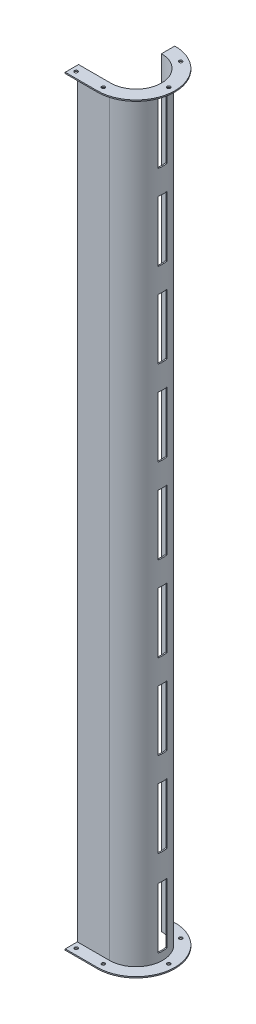
SolidWorks part; units mm, degrees
ref_plane "前视" through (0, 0, 0) normal (0, 0, 1) x (1, 0, 0)
ref_plane "上视" through (0, 0, 0) normal (0, 1, 0) x (1, 0, 0)
ref_plane "右视" through (0, 0, 0) normal (1, 0, 0) x (0, 0, -1)
sketch "草图1" plane through (0, 0, 0) normal (0, 1, 0) x (1, 0, 0)
  line L0 (0, 0) -> (59.4065, 0) construction
  line L1 (0, 0) -> (0, 69.9008) construction
  line L2 (0, 0) -> (53, 0)
  line L3 (53, 0) -> (53, 88.0268) construction
  line L4 (0, -2) -> (53, -2)
  line L5 (53, 86) -> (53, 84)
  line L6 (0, 0) -> (0, -2)
  arc A0 (53, 0) -> (53, 84) centre (53, 42) ccw
  arc A1 (53, -2) -> (53, 86) centre (53, 42) ccw
  point P6 (42.0774, 56.8644)
  point P8 (0, 44)
  point P9 (40.1648, 56.2796)
  point P10 (0, 44)
  dimension "D3" = 2
  dimension "D2" = 42
  dimension "D1" = 53
extrude "凸台-拉伸1" add sketch "草图1" along normal blind 1256
sketch "草图3" plane through (0, 1256, 0) normal (0, 1, 0) x (1, 0, 0)
  line L0 (0, 0) -> (91.5194, 0) construction
  line L1 (0, 0) -> (53, 0)
  line L2 (53, 84) -> (53, 106)
  line L4 (0, -22) -> (53, -22)
  line L5 (0, 0) -> (0, -22)
  line L6 (54.8577, 105.973) -> (43.3453, 107.7442) construction
  line L7 (53, 84) -> (40, 86) construction
  arc A0 (53, 0) -> (53, 84) centre (53, 42) ccw
  arc A1 (53, -22) -> (53, 106) centre (53, 42) ccw
  arc A2 (53, -22) -> (54.8577, 105.973) centre (53, 42) ccw construction
  dimension "D1" = 22
extrude "凸台-拉伸2" add sketch "草图3" against normal blind 2
sketch "草图4" plane through (0, 0, 0) normal (0, -1, 0) x (1, 0, 0)
  line L0 (53, 0) -> (0, 0) construction
  line L1 (53, -106) -> (53, -86) construction
  line L2 (53, -86) -> (53, -84) construction
  line L3 (0, 22) -> (53, 22) construction
  line L4 (0, 2) -> (0, 22) construction
  line L5 (0, 0) -> (0, 2) construction
  line L6 (53, 0) -> (0, 0)
  line L7 (53, -106) -> (53, -86)
  line L8 (53, -86) -> (53, -84)
  line L9 (0, 22) -> (53, 22)
  line L10 (0, 2) -> (0, 22)
  line L11 (0, 0) -> (0, 2)
  arc A0 (53, -84) -> (53, 0) centre (53, -42) ccw construction
  arc A1 (53, -106) -> (53, 22) centre (53, -42) ccw construction
  arc A2 (53, -84) -> (53, 0) centre (53, -42) ccw
  arc A3 (53, -106) -> (53, 22) centre (53, -42) ccw
extrude "凸台-拉伸3" add sketch "草图4" against normal blind 2
sketch "草图5" plane through (0, 0, 0) normal (1, 0, 0) x (0, 0, -1)
  line L0 (0, 0) -> (0, 95.5801) construction
  line L1 (0, 1256) -> (0, 0) construction
  line L2 (0, 0) -> (141.4525, 0) construction
  line L3 (-2, 1254) -> (86, 1254) construction
  line L4 (34.75, 115.4213) -> (49.75, 115.4213)
  line L5 (34.75, 115.4213) -> (34.75, 15.4213)
  line L6 (34.75, 15.4213) -> (49.75, 15.4213)
  line L7 (49.75, 115.4213) -> (49.75, 15.4213)
  line L8 (106, 2) -> (-22, 2) construction
  line L9 (42, 2) -> (42, 1357.7119) construction
  line L10 (34.75, 258) -> (49.75, 258)
  line L11 (86, 2) -> (-2, 2) construction
  line L12 (34.75, 258) -> (34.75, 158)
  line L13 (34.75, 158) -> (49.75, 158)
  line L14 (49.75, 258) -> (49.75, 158)
  line L15 (34.75, 998) -> (49.75, 998)
  line L16 (34.75, 998) -> (34.75, 1098)
  line L17 (34.75, 1098) -> (49.75, 1098)
  line L18 (49.75, 998) -> (49.75, 1098)
  line L19 (34.75, 398) -> (49.75, 398)
  line L20 (34.75, 398) -> (34.75, 298)
  line L21 (34.75, 298) -> (49.75, 298)
  line L22 (49.75, 398) -> (49.75, 298)
  line L23 (34.75, 538) -> (49.75, 538)
  line L24 (34.75, 538) -> (34.75, 438)
  line L25 (34.75, 438) -> (49.75, 438)
  line L26 (49.75, 538) -> (49.75, 438)
  line L27 (34.75, 678) -> (49.75, 678)
  line L28 (34.75, 678) -> (34.75, 578)
  line L29 (34.75, 578) -> (49.75, 578)
  line L30 (49.75, 678) -> (49.75, 578)
  line L31 (34.75, 818) -> (49.75, 818)
  line L32 (34.75, 818) -> (34.75, 718)
  line L33 (34.75, 718) -> (49.75, 718)
  line L34 (49.75, 818) -> (49.75, 718)
  line L35 (34.75, 958) -> (49.75, 958)
  line L36 (34.75, 958) -> (34.75, 858)
  line L37 (34.75, 858) -> (49.75, 858)
  line L38 (49.75, 958) -> (49.75, 858)
  line L39 (34.75, 1138) -> (49.75, 1138)
  line L40 (34.75, 1138) -> (34.75, 1238)
  line L41 (34.75, 1238) -> (49.75, 1238)
  line L42 (49.75, 1138) -> (49.75, 1238)
  dimension "D1" = 100
  dimension "D2" = 15
  dimension "D3" = 7.25
  dimension "D4" = 40
  dimension "D5" = 100
  dimension "D6" = 40
  dimension "D7" = 100
  dimension "D8" = 40
  dimension "D9" = 100
  dimension "D10" = 40
  dimension "D11" = 100
  dimension "D12" = 40
  dimension "D13" = 100
  dimension "D14" = 40
  dimension "D15" = 100
  dimension "D16" = 40
  dimension "D17" = 100
  dimension "D18" = 16
  dimension "D19" = 13.4213
extrude "切除-拉伸2" cut sketch "草图5" along normal blind 265
sketch "草图6" plane through (0, 1256, 0) normal (0, 1, 0) x (1, 0, 0)
  line L0 (53, 42) -> (81.375, 91.1469) construction
  line L1 (53, 106) -> (53, 84) construction
  line L2 (53, -12) -> (-21.8051, -12) construction
  circle A0 centre (53, 42) radius 54 construction
  circle A1 centre (80, 88.7654) radius 2.75
  circle A2 centre (107, 42) radius 2.75
  circle A3 centre (53, -12) radius 2.75
  circle A4 centre (8, -12) radius 2.75
  dimension "D1" = 108
  dimension "D2" = 5.5
  dimension "D3" = 5.5
  dimension "D4" = 5.5
  dimension "D6" = 5.5
  dimension "D7" = 45
  dimension "D5" = 30
extrude "切除-拉伸3" cut sketch "草图6" against normal blind 1510
